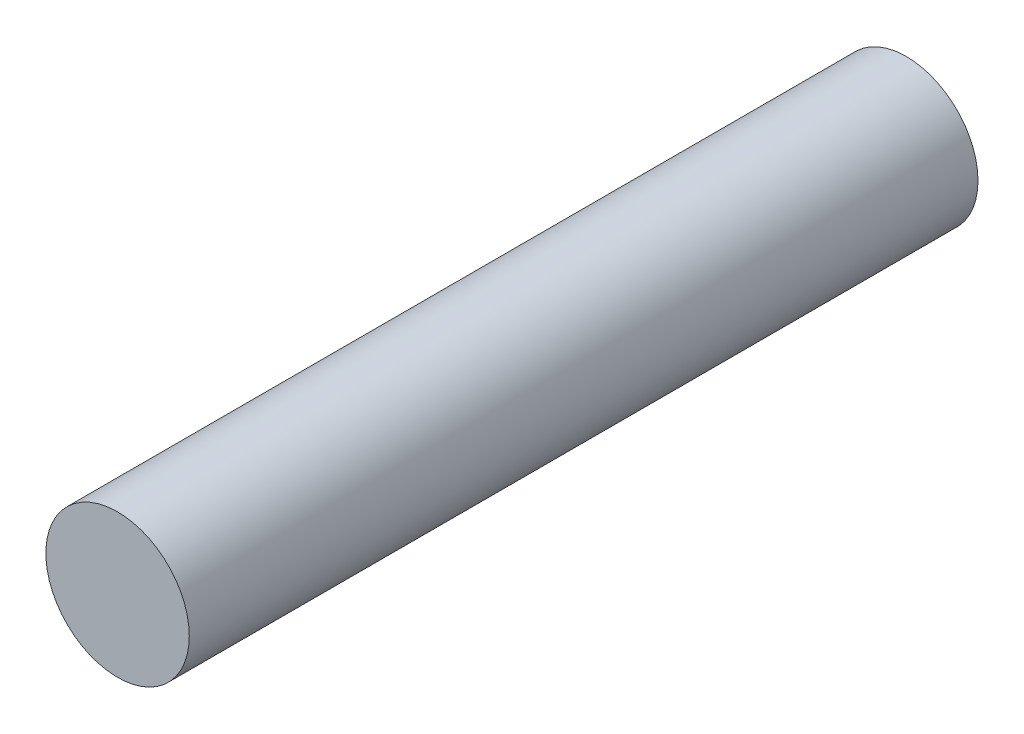
SolidWorks part; units mm, degrees
ref_plane "Front Plane" through (0, 0, 0) normal (0, 0, 1) x (1, 0, 0)
ref_plane "Top Plane" through (0, 0, 0) normal (0, 1, 0) x (1, 0, 0)
ref_plane "Right Plane" through (0, 0, 0) normal (1, 0, 0) x (0, 0, -1)
sketch "Sketch1" plane through (0, 0, 0) normal (0, 0, 1) x (1, 0, 0)
  circle A0 centre (0, 0) radius 5
  dimension "D1" = 10
extrude "Boss-Extrude1" add sketch "Sketch1" along normal blind 55
